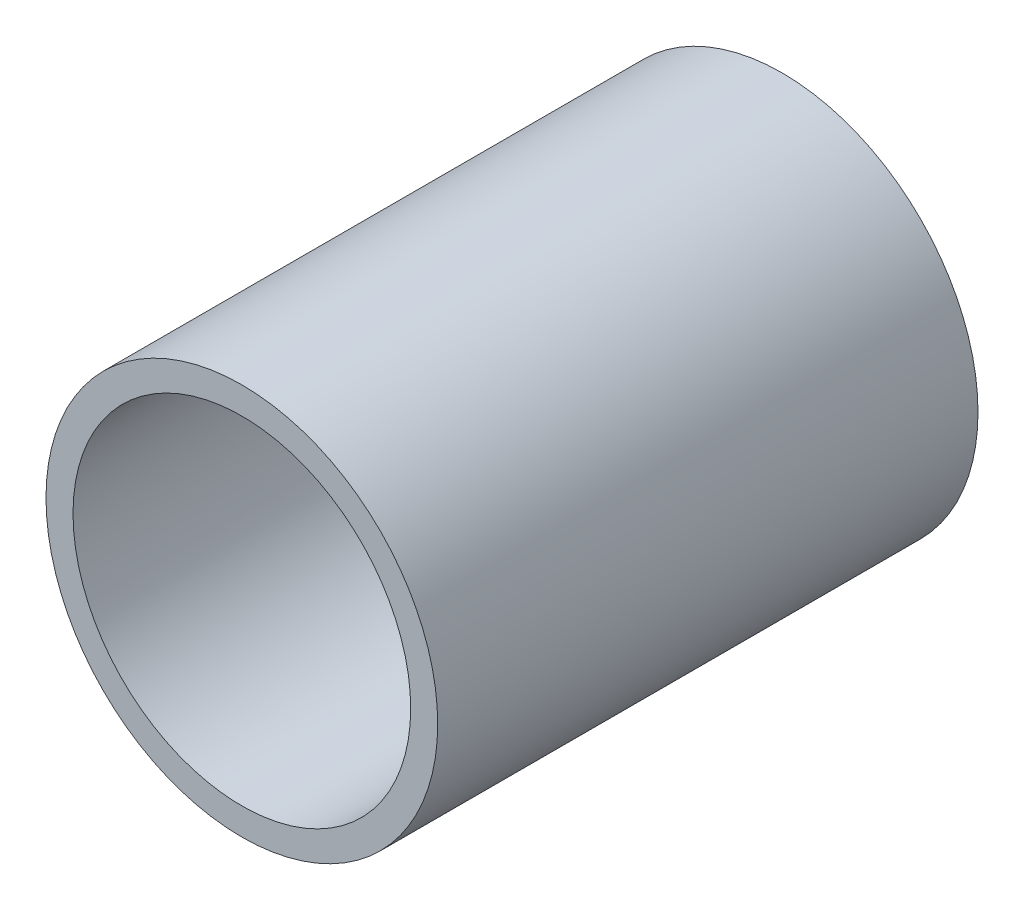
SolidWorks part; units mm, degrees
material "Q235A"
ref_plane "Front Plane" through (0, 0, 0) normal (0, 0, 1) x (1, 0, 0)
ref_plane "Top Plane" through (0, 0, 0) normal (0, 1, 0) x (1, 0, 0)
ref_plane "Right Plane" through (0, 0, 0) normal (1, 0, 0) x (0, 0, -1)
sketch "Sketch1" plane through (0, 0, 0) normal (0, 0, 1) x (1, 0, 0)
  circle A0 centre (0, 0) radius 14.5
  circle A1 centre (0, 0) radius 12.5
  dimension "D1" = 25
  dimension "D2" = 29
extrude "Boss-Extrude1" add sketch "Sketch1" along normal blind 40
